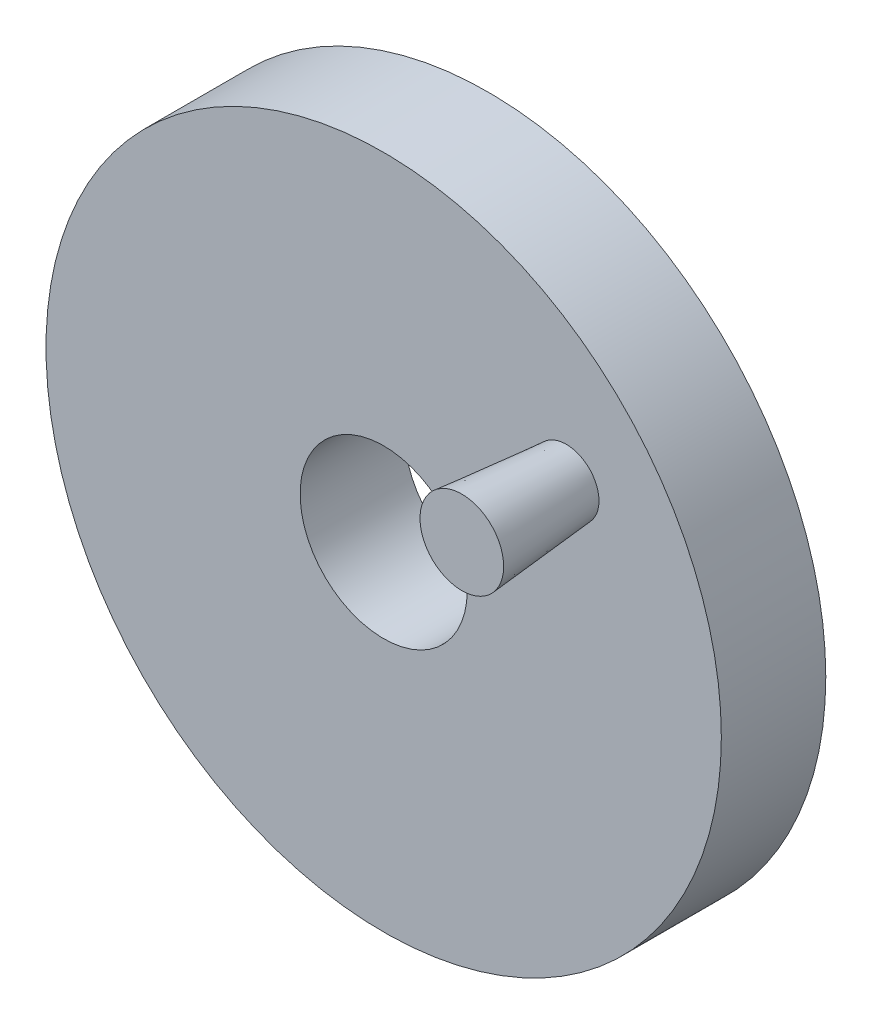
SolidWorks part; units mm, degrees
ref_plane "Front Plane" through (0, 0, 0) normal (0, 0, 1) x (1, 0, 0)
ref_plane "Top Plane" through (0, 0, 0) normal (0, 1, 0) x (1, 0, 0)
ref_plane "Right Plane" through (0, 0, 0) normal (1, 0, 0) x (0, 0, -1)
sketch "Sketch1" plane through (0, 0, 0) normal (0, 0, 1) x (1, 0, 0)
  circle A0 centre (0, -208.7074) radius 32.3276
  circle A1 centre (0, -208.7074) radius 8
extrude "Boss-Extrude1" add sketch "Sketch1" against normal blind 10
sketch "Sketch2" plane through (0, 0, 0) normal (0, 0, 1) x (1, 0, 0)
  circle A0 centre (17.4821, -194.9769) radius 3.1297
extrude "Boss-Extrude2" add sketch "Sketch2" along normal blind 10 draft 5 draft outward yes
